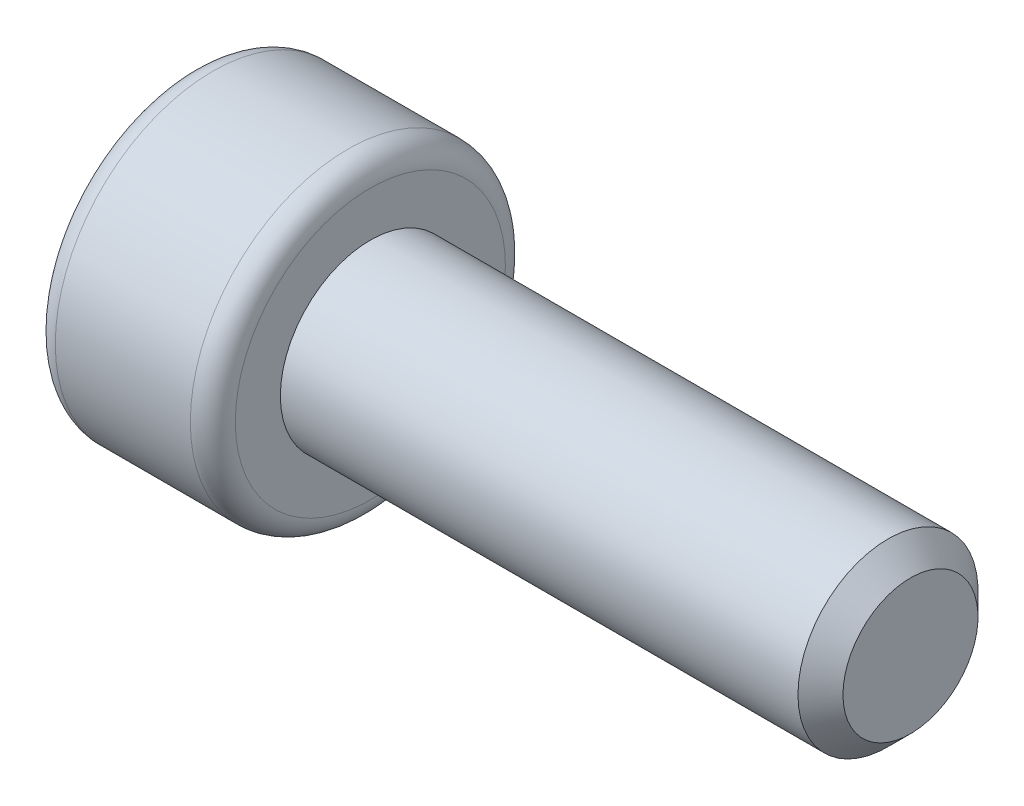
SolidWorks part; units mm, degrees
material "AISI 304"
ref_plane "Front Plane" through (0, 0, 0) normal (0, 0, 1) x (1, 0, 0)
ref_plane "Top Plane" through (0, 0, 0) normal (0, 1, 0) x (1, 0, 0)
ref_plane "Right Plane" through (0, 0, 0) normal (1, 0, 0) x (0, 0, -1)
sketch "Sketch1" plane through (0, 0, 0) normal (0, 0, 1) x (1, 0, 0)
  line L0 (-4.7092, 0) -> (16, 0) construction
  line L1 (0, 0) -> (0, 3.5)
  line L2 (0, 3.5) -> (4, 3.5)
  line L3 (4, 3.5) -> (4, 2)
  line L4 (4, 2) -> (16, 2)
  line L5 (16, 2) -> (16, 0)
  line L6 (16, 0) -> (0, 0)
  dimension "D1" = 7
  dimension "D2" = 4
  dimension "D3" = 4
  dimension "D4" = 12
revolve "Revolve1" add sketch "Sketch1" angle 360 about L0
cosmetic thread "Cosmetic Thread1" parameters "D2"=3
sketch "Sketch4" plane through (0, 0, 0) normal (-1, 0, 0) x (0, 0, 1)
  line L1 (-1.7321, 0) -> (-0.866, -1.5)
  line L2 (-0.866, -1.5) -> (0.866, -1.5)
  line L3 (0.866, -1.5) -> (1.7321, 0)
  line L4 (1.7321, 0) -> (0.866, 1.5)
  line L5 (0.866, 1.5) -> (-0.866, 1.5)
  line L6 (-0.866, 1.5) -> (-1.7321, 0)
  circle A0 centre (0, 0) radius 1.5 construction
extrude "Cut-Extrude1" cut sketch "Sketch4" against normal blind 2
fillet "Fillet1" radius 0.5 2 edges at (4, 0, 3.5) (0, 0, 3.5)
chamfer "Chamfer1" distance 0.1 angle 80 6 edges at (0, -0.75, -1.299) (0, -1.5, 0) (0, -0.75, 1.299) (0, 0.75, 1.299) (0, 1.5, 0) (0, 0.75, -1.299)
chamfer "Chamfer2" distance 0.5 angle 45 1 edges at (16, 0, 2)
